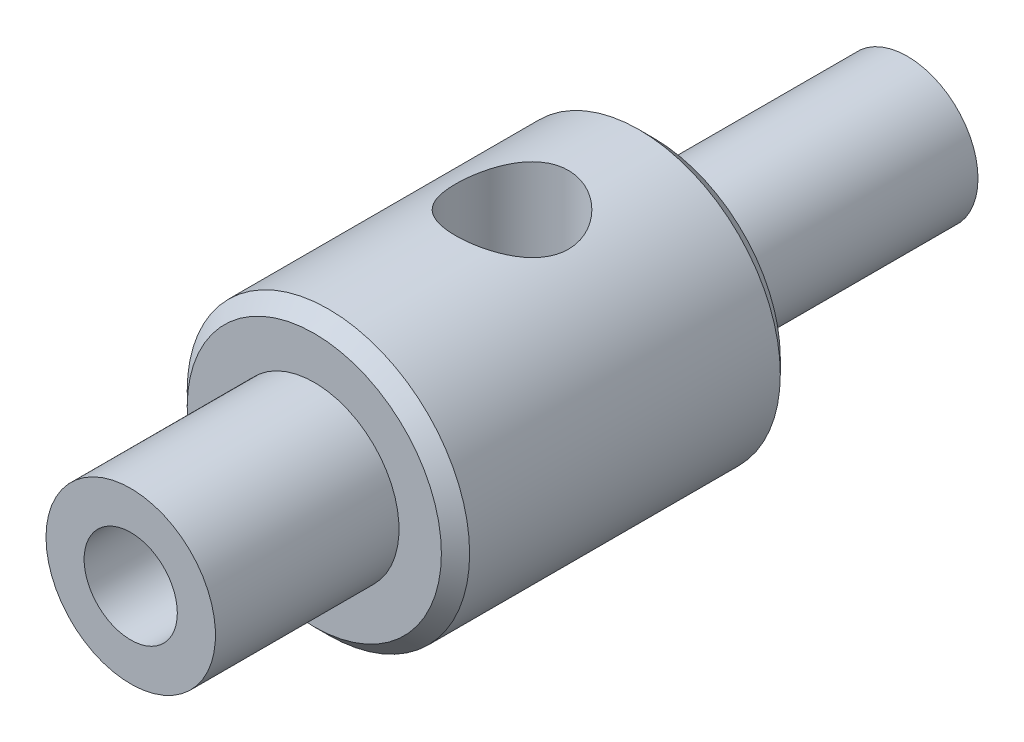
from build123d import *

# Parameters (mm, degrees)
SKETCH1_R             = 5
BOSS_EXTRUDE1_DEPTH   = 12
SKETCH2_R             = 3
BOSS_EXTRUDE2_DEPTH   = 6.5
M4_TAPPED_HOLE1_D     = 3.3
M4_TAPPED_HOLE1_DEPTH = 10.1
M4_TAPPED_HOLE1_TIP   = 0.991420021
SKETCH5_R             = 2.5
BOSS_EXTRUDE3_DEPTH   = 9
SKETCH6_R             = 2
CUT_EXTRUDE1_DEPTH    = 7.5
CHAMFER1_SIZE         = 0.5


with BuildPart() as part:
    # Sketch1 → Boss-Extrude1 (new body)
    with BuildSketch(Plane.XY):
        Circle(SKETCH1_R)
    extrude(amount=BOSS_EXTRUDE1_DEPTH)

    # Sketch2 → Boss-Extrude2 (add)
    with BuildSketch(Plane.XY.offset(12)):
        with Locations(Location((0, 0, 0), (0, 0, 180))):
            Circle(SKETCH2_R)
    extrude(amount=BOSS_EXTRUDE2_DEPTH)

    # M4 Tapped Hole1
    with Locations(Plane.XY.offset(18.5)):
        with Locations((0, 0)):
            Hole(M4_TAPPED_HOLE1_D / 2, depth=M4_TAPPED_HOLE1_DEPTH)
            with Locations((0, 0, -(M4_TAPPED_HOLE1_DEPTH + M4_TAPPED_HOLE1_TIP / 2))):  # 118° drill point
                Cone(0, M4_TAPPED_HOLE1_D / 2, M4_TAPPED_HOLE1_TIP, mode=Mode.SUBTRACT)

    # Sketch5 → Boss-Extrude3 (add)
    with BuildSketch(Plane(origin=(0, 0, 0), x_dir=(-1, 0, 0), z_dir=(0, 0, -1))):
        with Locations(Location((0, 0, 0), (0, 0, 180))):
            Circle(SKETCH5_R)
    extrude(amount=BOSS_EXTRUDE3_DEPTH)

    # Sketch6 → Cut-Extrude1 (cut, symmetric)
    with BuildSketch(Plane(origin=(0, 0, 0), x_dir=(1, 0, 0), z_dir=(0, 1, 0))):
        with Locations(Location((0, -5, 0), (0, 0, 270))):
            Circle(SKETCH6_R)
    extrude(amount=CUT_EXTRUDE1_DEPTH, both=True, mode=Mode.SUBTRACT)

    # Chamfer1
    chamfer1_edges = [part.edges().sort_by_distance(p)[0] for p in [
        (-5, 0, 0),
        (-5, 0, 12),
    ]]
    chamfer(chamfer1_edges, length=CHAMFER1_SIZE)


solid = part.part
